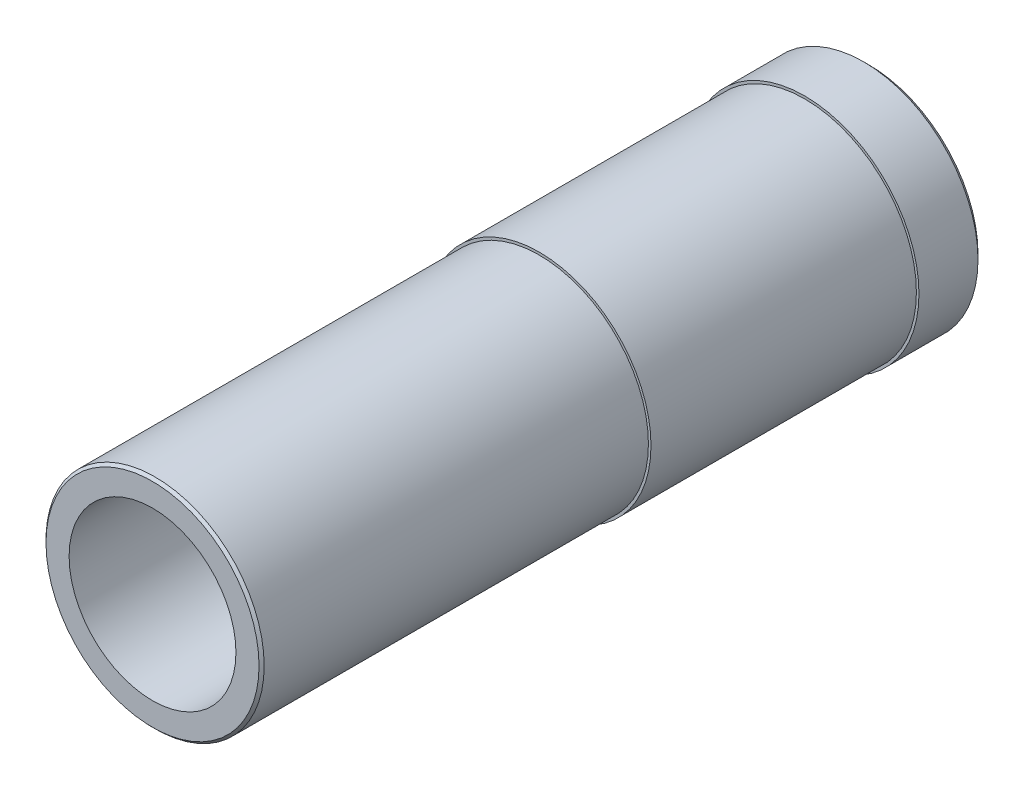
SolidWorks part; units mm, degrees
material "普通碳钢"
ref_plane "前视基准面" through (0, 0, 0) normal (0, 0, 1) x (1, 0, 0)
ref_plane "上视基准面" through (0, 0, 0) normal (0, 1, 0) x (1, 0, 0)
ref_plane "右视基准面" through (0, 0, 0) normal (1, 0, 0) x (0, 0, -1)
sketch "草图1" plane through (0, 0, 0) normal (0, 0, 1) x (1, 0, 0)
  circle A0 centre (0, 0) radius 44.5
  circle A1 centre (0, 0) radius 32.5
  dimension "D1" = 89
  dimension "D2" = 65
extrude "凸台-拉伸1" add sketch "草图1" along normal blind 279.1
ref_plane "基准面1" through (0, 0, 25) normal (0, 0, -1) x (-1, 0, 0)
sketch "草图2" plane through (0, 0, 25) normal (0, 0, -1) x (-1, 0, 0)
  circle A0 centre (0, 0) radius 44.5
  circle A1 centre (0, 0) radius 43.5
  dimension "D1" = 89
  dimension "D2" = 87
extrude "切除-拉伸1" cut sketch "草图2" against normal up to surface (254.1 mm away) up to face at (44.5, 0, 279.1)
sketch "草图3" plane through (0, 0, 279.1) normal (0, 0, 1) x (1, 0, 0)
  circle A0 centre (0, 0) radius 43.5
  circle A1 centre (0, 0) radius 42.5
  dimension "D1" = 87
  dimension "D2" = 85
extrude "切除-拉伸2" cut sketch "草图3" against normal blind 150.7
chamfer "倒角1" distance 2 angle 45 1 edges at (44.5, 0, 0)
chamfer "倒角2" distance 1 angle 45 1 edges at (42.5, 0, 279.1)
